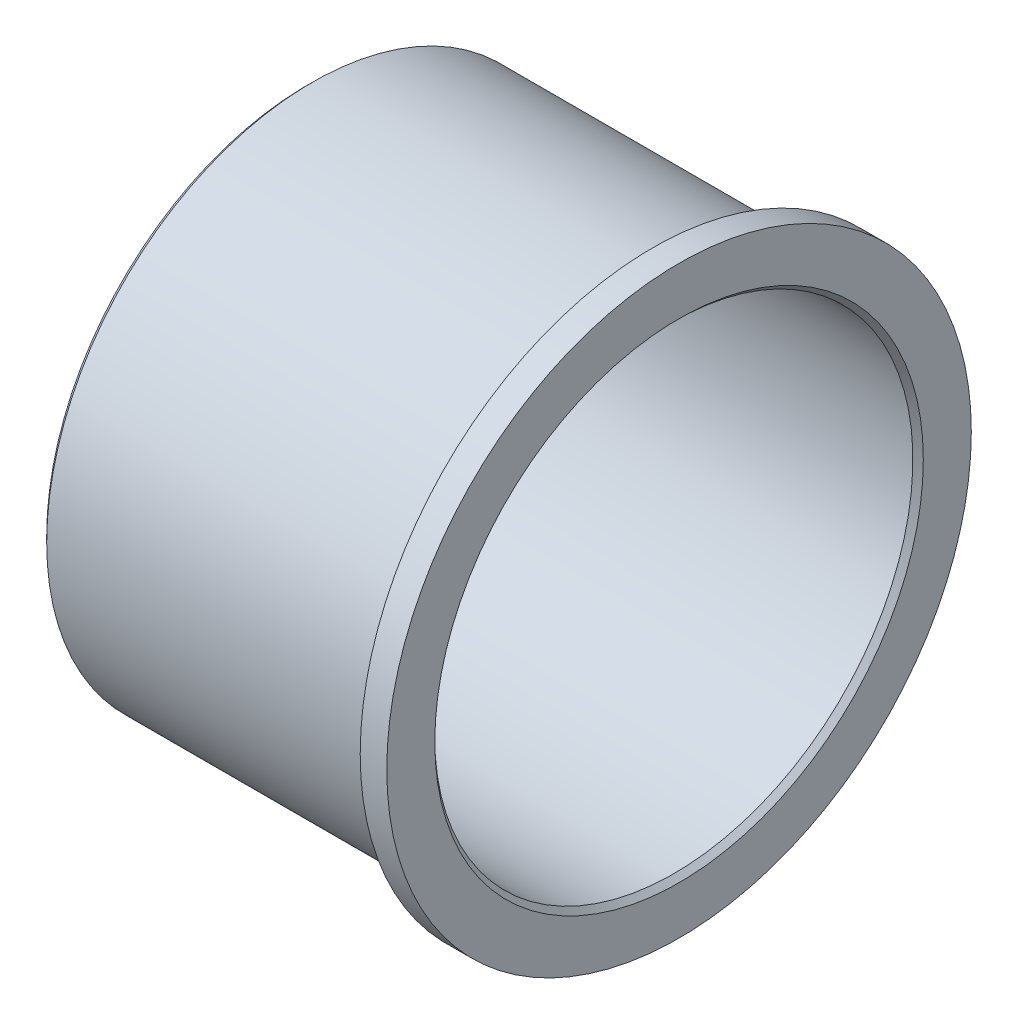
from build123d import *


with BuildPart() as part:
    # Sketch 181 → 旋转1 (revolve)
    with BuildSketch(Plane.XY, mode=Mode.PRIVATE) as revolve_1_sk:
        Polygon((-35, 45.965688775), (-34, 45), (34, 45), (35, 45.965688775), (35, 55), (30, 55), (30, 49.8), (28, 49.8), (28, 50), (-34, 50), (-35, 49), align=None)
    revolve(revolve_1_sk.sketch.rotate(Axis((-35, 0, 0), (1, 0, 0)), 90), axis=Axis((-35, 0, 0), (1, 0, 0)))


solid = part.part
